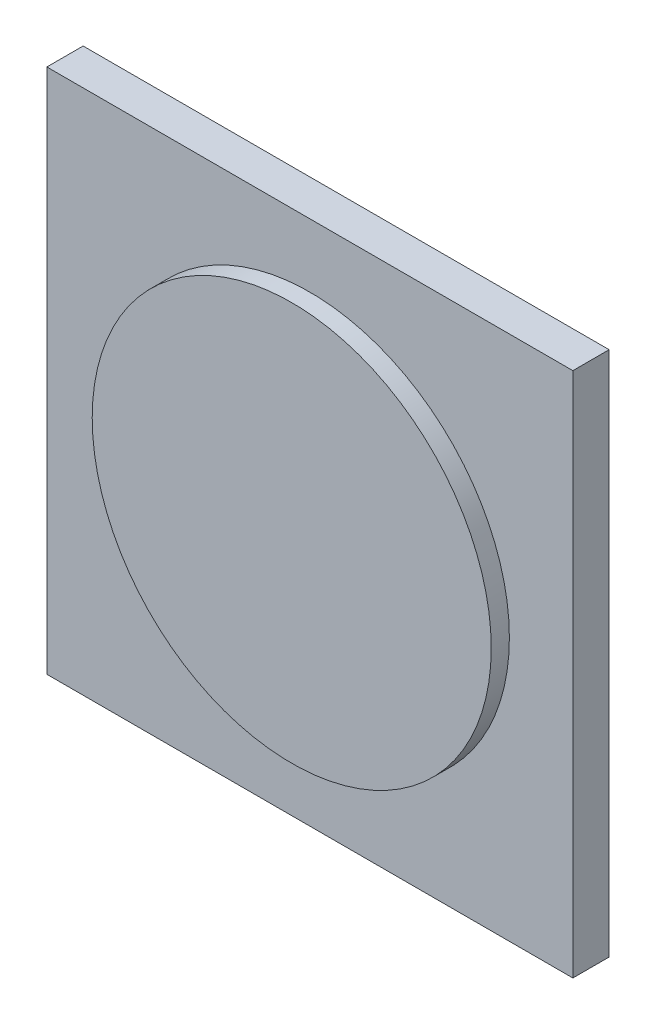
from build123d import *

# Parameters (mm, degrees)
SKETCH1_W           = 145
SKETCH1_H           = 145
BOSS_EXTRUDE1_DEPTH = 10
SKETCH2_R           = 55
BOSS_EXTRUDE2_DEPTH = 5


with BuildPart() as part:
    # Sketch1 → Boss-Extrude1 (new body)
    with BuildSketch(Plane.XY):
        with Locations((72.5, 72.5)):
            Rectangle(SKETCH1_W, SKETCH1_H)
    extrude(amount=BOSS_EXTRUDE1_DEPTH)

    # Sketch2 → Boss-Extrude2 (add)
    with BuildSketch(Plane.XY.offset(10)):
        with Locations(Location((72.5, 72.5, 0), (0, 0, 180))):
            Circle(SKETCH2_R)
    extrude(amount=BOSS_EXTRUDE2_DEPTH)


solid = part.part
